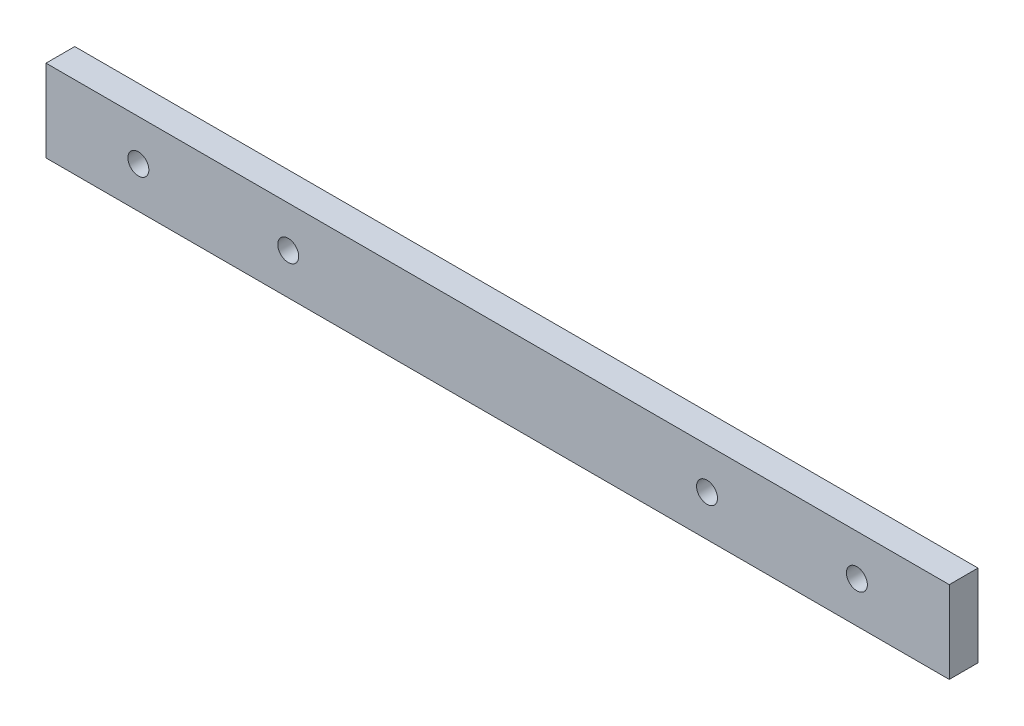
SolidWorks part; units mm, degrees
material "普通碳钢"
ref_plane "前视基准面" through (0, 0, 0) normal (0, 0, 1) x (1, 0, 0)
ref_plane "上视基准面" through (0, 0, 0) normal (0, 1, 0) x (1, 0, 0)
ref_plane "右视基准面" through (0, 0, 0) normal (1, 0, 0) x (0, 0, -1)
sketch "草图1" plane through (0, 0, 0) normal (0, 0, 1) x (1, 0, 0)
  line L1 (0, 0) -> (440, 0)
  line L2 (0, 0) -> (0, 40)
  line L3 (0, 40) -> (440, 40)
  line L4 (440, 0) -> (440, 40)
  dimension "D1" = 40
  dimension "D2" = 440
extrude "凸台-拉伸1" add sketch "草图1" along normal blind 14
hole_wizard "M12 螺纹孔1" positions "3D草图1" profile "草图2" tap size "M12" standard "GB"
sketch3d "3D草图1"
  line L0 (0, 20, 14) -> (440, 20, 14) construction
  line L1 (0, 40, 14) -> (0, 0, 14) construction
  line L2 (440, 0, 14) -> (440, 40, 14) construction
  point P0 (45, 20, 14)
  point P2 (118, 20, 14)
  point P4 (395, 20, 14)
  point P6 (322, 20, 14)
  dimension "D1" = 73
  dimension "D2" = 73
  dimension "D3" = 277
  dimension "D4" = 45
sketch "草图2" plane through (45, 20, 14) normal (1, 0, 0) x (0, -1, 0)
  line L0 (0, 0) -> (0, 32.3144)
  line L1 (0, 32.3144) -> (5.1, 29.25)
  line L2 (5.1, 29.25) -> (5.1, 0)
  line L5 (5.1, 0) -> (0, 0)
  line L10 (0, 32.3144) -> (-5.1, 29.25) construction
  line L11 (0, -6.35) -> (0, 107.95) construction
  dimension "螺纹孔钻头直径" = 10.2
  dimension "螺纹孔钻头深度" = 29.25
  dimension "导头角度" = 118
cosmetic thread "孔螺蚊线1"
cosmetic thread "孔螺蚊线2"
cosmetic thread "孔螺蚊线3"
cosmetic thread "孔螺蚊线4"
